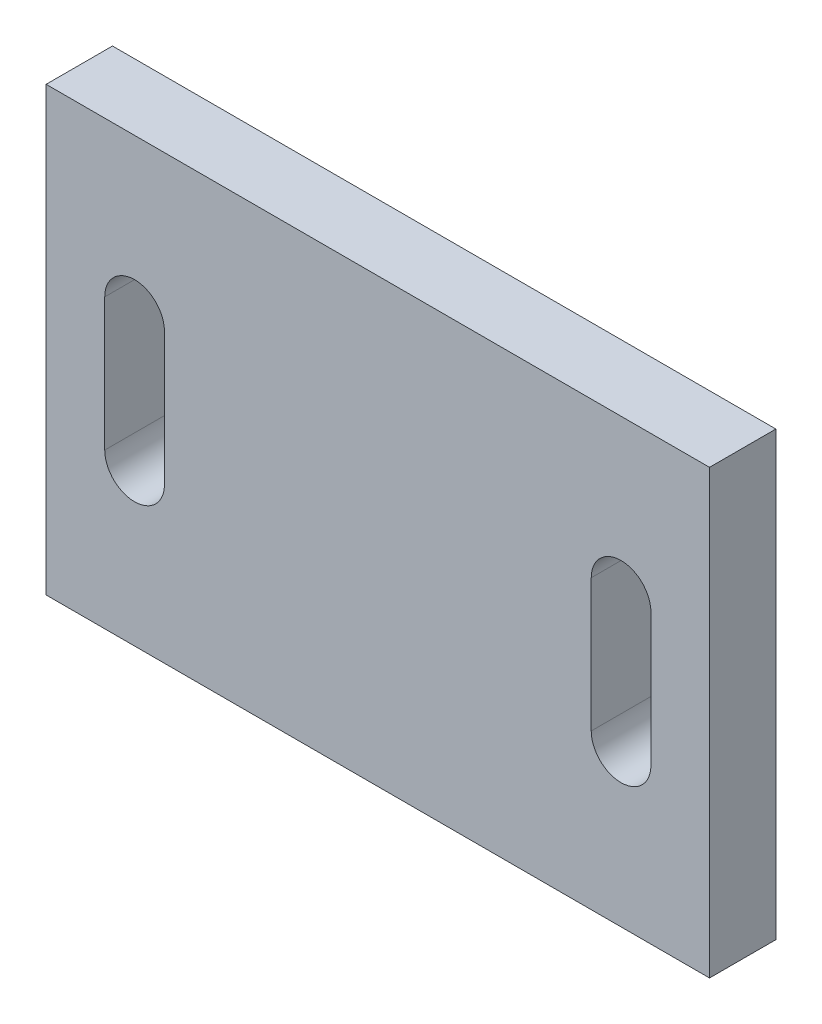
SolidWorks part; units mm, degrees
material "Q235B"
ref_plane "Front Plane" through (0, 0, 0) normal (0, 0, 1) x (1, 0, 0)
ref_plane "Top Plane" through (0, 0, 0) normal (0, 1, 0) x (1, 0, 0)
ref_plane "Right Plane" through (0, 0, 0) normal (1, 0, 0) x (0, 0, -1)
sketch "Sketch1" plane through (0, 0, 0) normal (0, 0, 1) x (1, 0, 0)
  line L0 (260, 130) -> (260, 70) construction
  line L1 (0, 0) -> (300, 0)
  line L2 (0, 0) -> (0, 200)
  line L3 (0, 200) -> (300, 200)
  line L4 (300, 0) -> (300, 200)
  line L5 (273.5, 130) -> (273.5, 70)
  line L6 (246.5, 130) -> (246.5, 70)
  line L7 (40, 130) -> (40, 70) construction
  line L8 (53.5, 130) -> (53.5, 70)
  line L9 (26.5, 130) -> (26.5, 70)
  arc A0 (273.5, 130) -> (246.5, 130) centre (260, 130) ccw
  arc A1 (246.5, 70) -> (273.5, 70) centre (260, 70) ccw
  arc A2 (53.5, 130) -> (26.5, 130) centre (40, 130) ccw
  arc A3 (26.5, 70) -> (53.5, 70) centre (40, 70) ccw
  point P7 (260, 100)
  point P12 (40, 100)
  dimension "D3" = 13.5
  dimension "D1" = 300
  dimension "D2" = 200
  dimension "D4" = 60
  dimension "D5" = 40
  dimension "D6" = 40
  dimension "D7" = 100
  dimension "D8" = 100
extrude "Boss-Extrude1" add sketch "Sketch1" along normal blind 30
